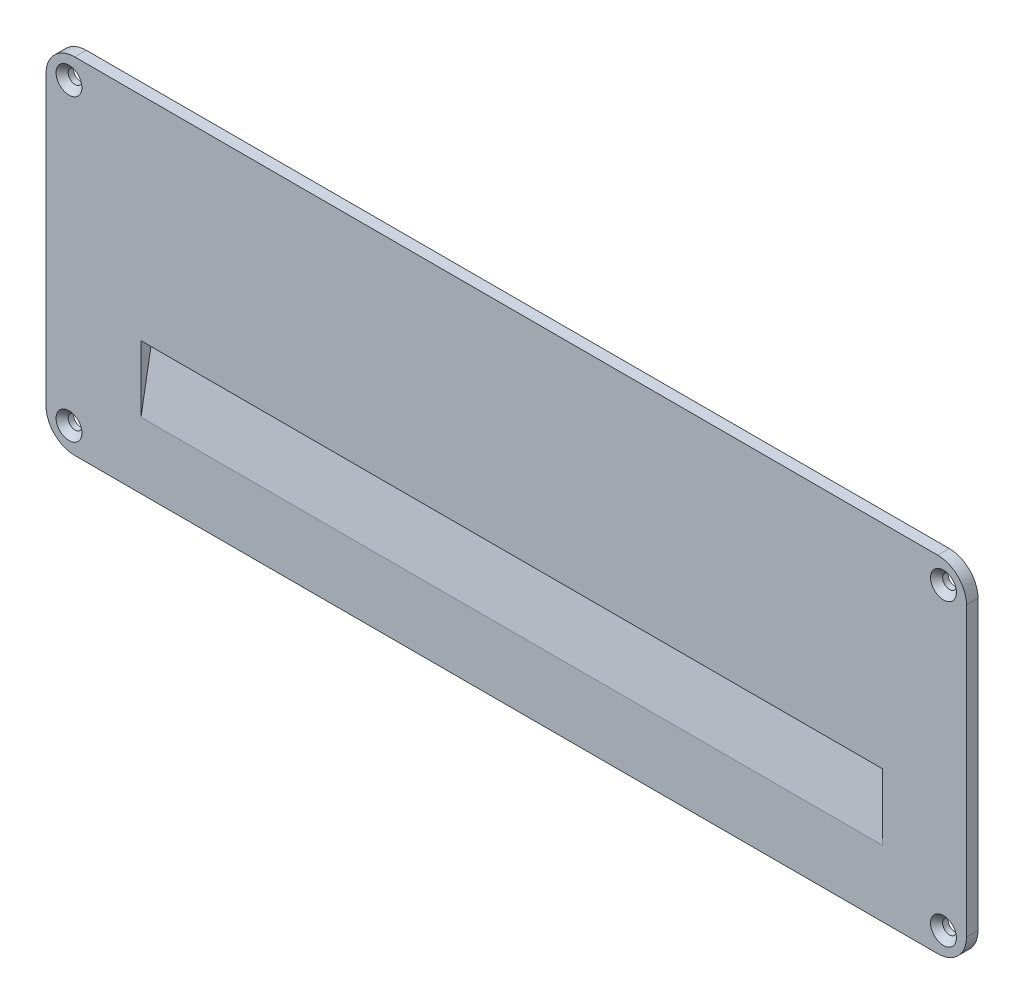
from build123d import *

# Parameters (mm, degrees)
SKETCH1_W                                         = 160
SKETCH1_H                                         = 60
BOSS_EXTRUDE1_DEPTH                               = 2
SKETCH2_R                                         = 0.5
CUT_EXTRUDE1_DEPTH                                = 2
PILOT_HOLE_SIZE_PER_CROSS_SLOTTED_COU_D           = 2.4
PILOT_HOLE_SIZE_PER_CROSS_SLOTTED_COU_DEPTH       = 7.5
PILOT_HOLE_SIZE_PER_CROSS_SLOTTED_COU_CSINK_D     = 4.5
PILOT_HOLE_SIZE_PER_CROSS_SLOTTED_COU_CSINK_ANGLE = 90
PILOT_HOLE_SIZE_PER_CROSS_SLOTTED_COU_TIP         = 0.721032743
SKETCH6_W                                         = 128.916628893
SKETCH6_H                                         = 2
CUT_EXTRUDE3_DEPTH                                = 100
FILLET1_R                                         = 5


with BuildPart() as part:
    # Sketch1 → Boss-Extrude1 (new body)
    with BuildSketch(Plane.XY):
        Rectangle(SKETCH1_W, SKETCH1_H)
    extrude(amount=BOSS_EXTRUDE1_DEPTH)

    # Sketch2 → Cut-Extrude1 (cut)
    with BuildSketch(Plane.XY.offset(2)):
        with Locations((-76, 26)):
            Circle(SKETCH2_R)
        with Locations(Location((76, 26, 0), (0, 0, 180))):
            Circle(SKETCH2_R)
        with Locations((76, -26)):
            Circle(SKETCH2_R)
        with Locations(Location((-76, -26, 0), (0, 0, 180))):
            Circle(SKETCH2_R)
    extrude(amount=-CUT_EXTRUDE1_DEPTH, mode=Mode.SUBTRACT)

    # Pilot hole size (% per cross) slotted countersunk wood screw type1
    with Locations(Plane.XY.offset(2)):
        with Locations((-76, 26), (76, 26), (76, -26), (-76, -26)):
            CounterSinkHole(PILOT_HOLE_SIZE_PER_CROSS_SLOTTED_COU_D / 2, PILOT_HOLE_SIZE_PER_CROSS_SLOTTED_COU_CSINK_D / 2, depth=PILOT_HOLE_SIZE_PER_CROSS_SLOTTED_COU_DEPTH, counter_sink_angle=PILOT_HOLE_SIZE_PER_CROSS_SLOTTED_COU_CSINK_ANGLE)
            with Locations((0, 0, -(PILOT_HOLE_SIZE_PER_CROSS_SLOTTED_COU_DEPTH + PILOT_HOLE_SIZE_PER_CROSS_SLOTTED_COU_TIP / 2))):  # 118° drill point
                Cone(0, PILOT_HOLE_SIZE_PER_CROSS_SLOTTED_COU_D / 2, PILOT_HOLE_SIZE_PER_CROSS_SLOTTED_COU_TIP, mode=Mode.SUBTRACT)

    # Sketch6 → Cut-Extrude3 (cut)
    with BuildSketch(Plane(origin=(0, -29.437409455, 5.190609529), x_dir=(1, 0, 0), z_dir=(0, -0.9848077530122086, 0.17364817766692736))):
        with Locations((0.971111813, -0.2388368)):
            Rectangle(SKETCH6_W, SKETCH6_H)
    extrude(amount=-CUT_EXTRUDE3_DEPTH, mode=Mode.SUBTRACT)

    # Fillet1
    fillet1_edges = [part.edges().sort_by_distance(p)[0] for p in [
        (80, -30, 1),
        (-80, -30, 1),
        (-80, 30, 1),
        (80, 30, 1),
    ]]
    fillet(fillet1_edges, radius=FILLET1_R)


solid = part.part
